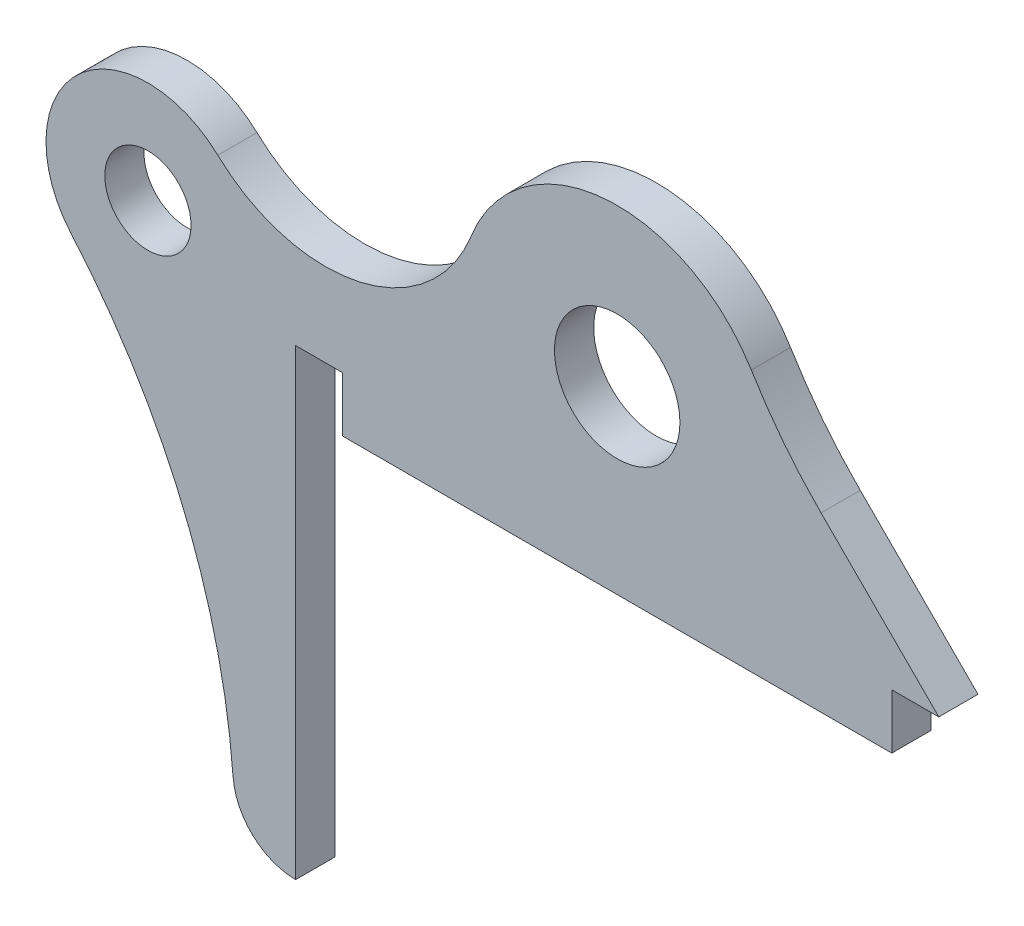
SolidWorks part; units mm, degrees
ref_plane "Front Plane" through (0, 0, 0) normal (0, 0, 1) x (1, 0, 0)
ref_plane "Top Plane" through (0, 0, 0) normal (0, 1, 0) x (1, 0, 0)
ref_plane "Right Plane" through (0, 0, 0) normal (1, 0, 0) x (0, 0, -1)
sketch "Sketch1" plane through (0, 0, 0) normal (0, 0, 1) x (1, 0, 0)
  line L0 (-175.1, -115) -> (175.1, -115)
  line L1 (-175.1, -115) -> (-175.1, -80)
  line L2 (-175.1, -80) -> (-205.1, -80)
  line L3 (-205.1, -80) -> (-205.1, -375)
  line L4 (175.1, -115) -> (175.1, -80)
  line L5 (175.1, -80) -> (205.1, -80)
  line L6 (205.1, -80) -> (130.0021, -4.9021)
  arc A0 (85.5335, 51.8075) -> (-93.0806, 36.5513) centre (0, 0) ccw
  arc A1 (-254.7302, 0.3131) -> (-348.4686, -89.5141) centre (-299.3, -47) ccw
  arc A2 (-254.7302, 0.3131) -> (-93.0806, 36.5513) centre (-186.1613, 73.1026) ccw
  arc A3 (-244.984, -338.0435) -> (-205.1, -375) centre (-205.1, -335) ccw
  arc A4 (-244.984, -338.0435) -> (-348.4686, -89.5141) centre (-673.7375, -370.7616) ccw
  arc A5 (85.5335, 51.8075) -> (130.0021, -4.9021) centre (342.1341, 207.23) ccw
  circle A6 centre (0, 0) radius 40
  circle A7 centre (-299.3, -47) radius 27.5
  dimension "D1" = 200
  dimension "D2" = 130
  dimension "D5" = 200
  dimension "D11" = 80
  dimension "D12" = 860
  dimension "D17" = 600
  dimension "D18" = 80
  dimension "D19" = 55
  dimension "D3" = 299.3
  dimension "D4" = 47
  dimension "D6" = 115
  dimension "D7" = 124.2
  dimension "D8" = 30
  dimension "D9" = 35
  dimension "D10" = 260
  dimension "D13" = 350.2
  dimension "D14" = 35
  dimension "D15" = 30
  dimension "D16" = 45
extrude "Boss-Extrude1" add sketch "Sketch1" along normal blind 25
